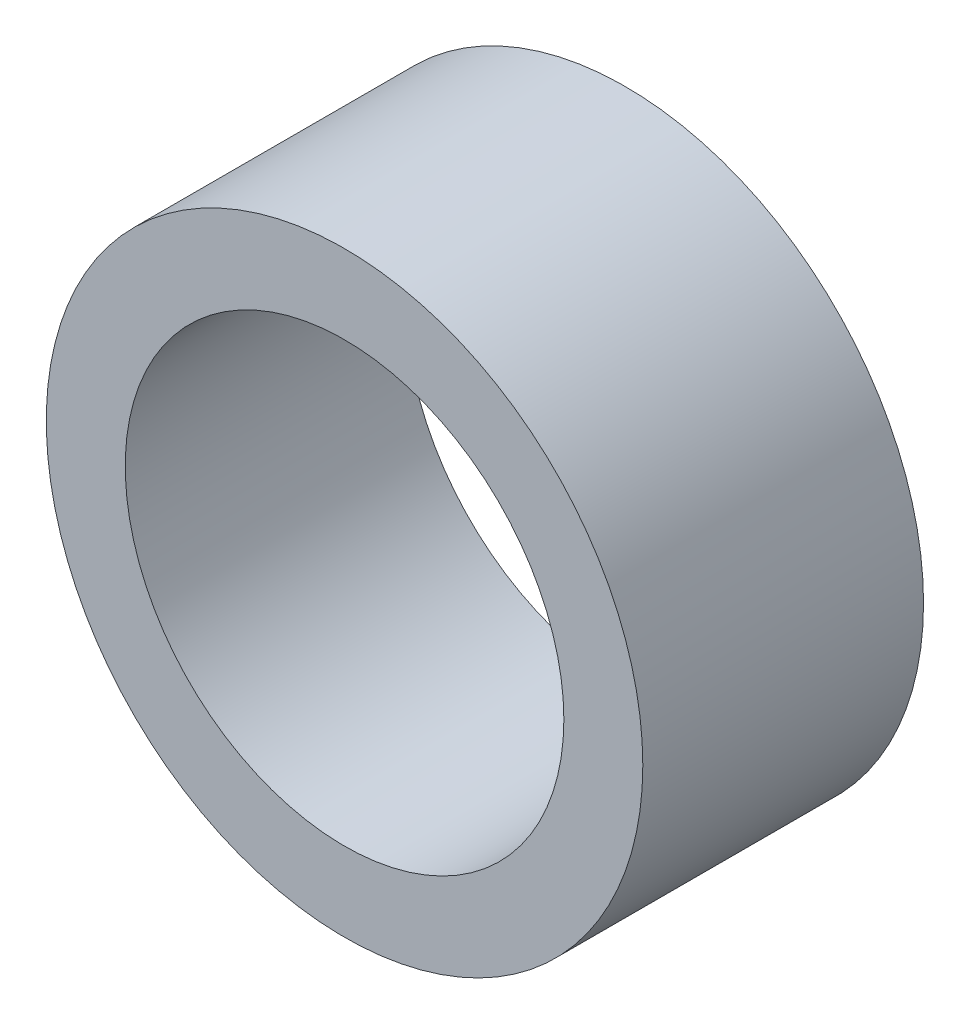
SolidWorks part; units mm, degrees
ref_plane "Front Plane" through (0, 0, 0) normal (0, 0, 1) x (1, 0, 0)
ref_plane "Top Plane" through (0, 0, 0) normal (0, 1, 0) x (1, 0, 0)
ref_plane "Right Plane" through (0, 0, 0) normal (1, 0, 0) x (0, 0, -1)
sketch "Sketch1" plane through (0, 0, 0) normal (0, 0, 1) x (1, 0, 0)
  circle A0 centre (0, 0) radius 8.5
  circle A1 centre (0, 0) radius 6.25
  dimension "D1" = 12.5
  dimension "D2" = 17
extrude "Boss-Extrude1" add sketch "Sketch1" along normal blind 8
